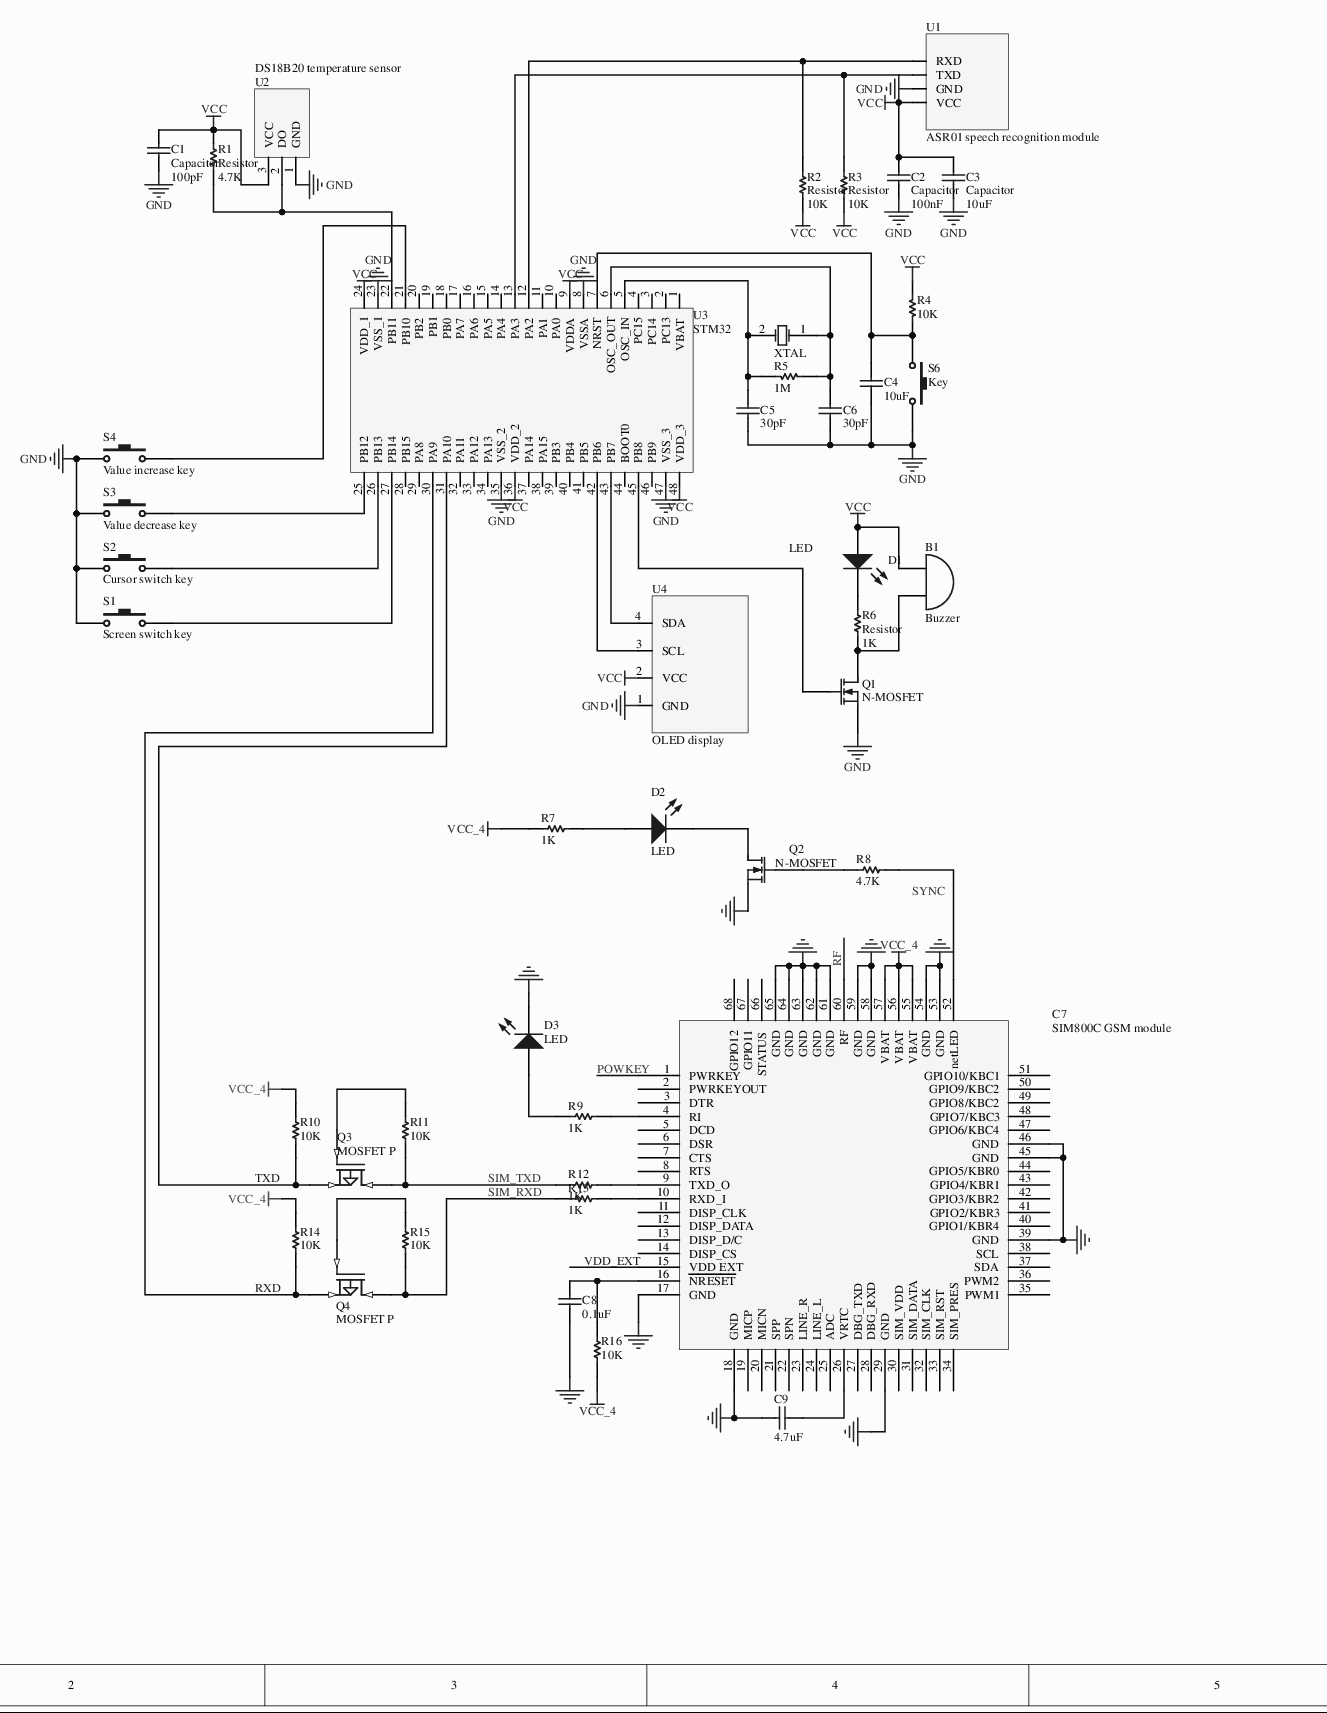
[diagram p0: MISC82701-2.SchDoc, left]
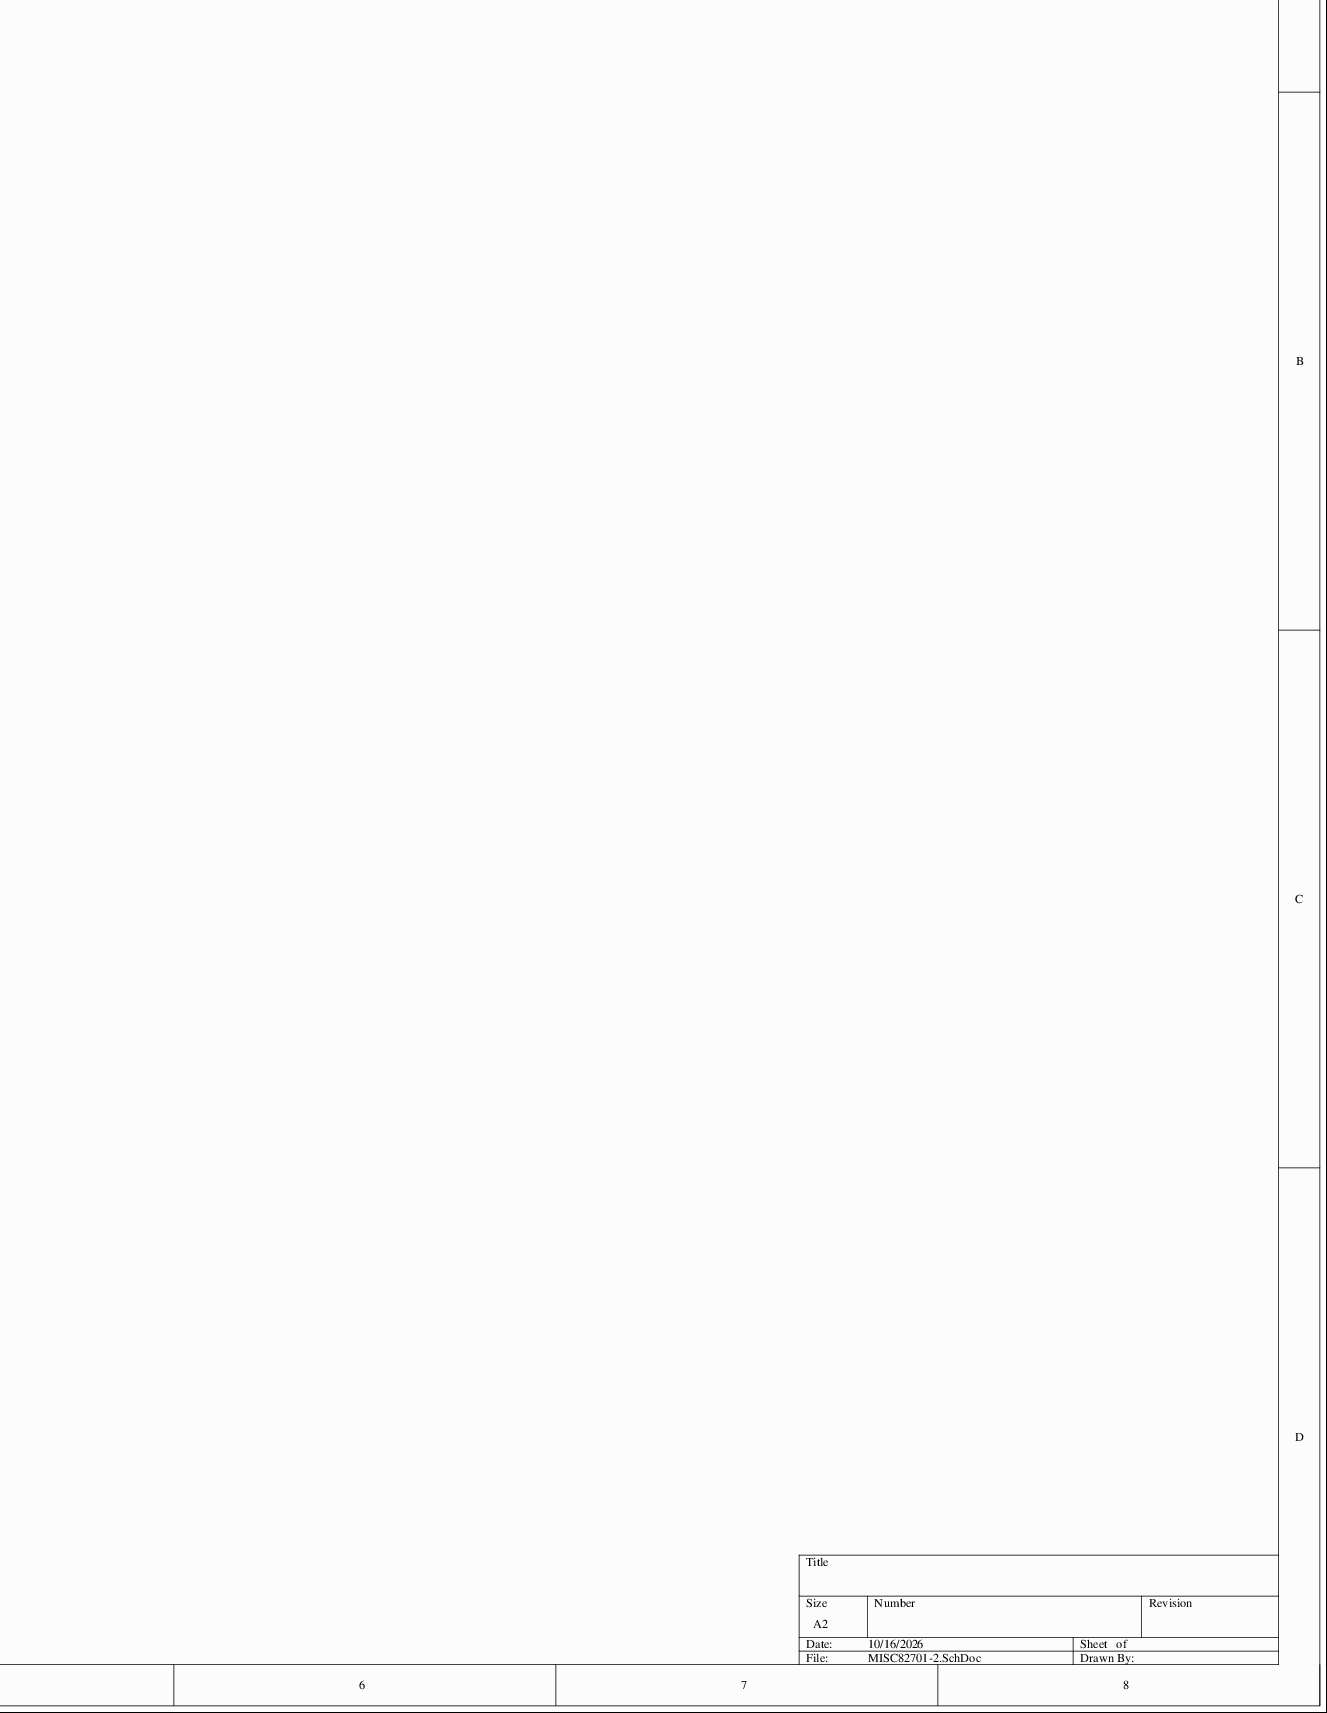
[diagram p1: MISC82701-2.SchDoc, right]
# Altium project MISC82701-7.PrjPcb
1 sheet, 43 parts. Net scope: global (net labels, ports and power ports of the same name join across sheets).
Board file: MISC82701.PcbDoc

## Sheet MISC82701-2.SchDoc
size A2

### Parts
B1  Buzzer  [PIN2]
C1  Capacitor  value 100pF  [0603C]
C2  Capacitor  value 100nF  [0603C]
C3  Capacitor  value 10uF  [0603C]
C4  10uF  [0603C]
C5  value 30pF  [0603C]  (hidden comment: Cap)
C6  value 30pF  [0603C]  (hidden comment: Cap)
C7  SIM800C GSM module  [GSMM_SMD_SIM900A]
C8  value 0.1uF  [0805C]  (hidden comment: Capacitor)
C9  value 4.7uF  [0805C]  (hidden comment: Capacitor)
D1  LED  [3.2X1.6X1.1]
D2  LED  [3.2X1.6X1.1]
D3  LED  [3.2X1.6X1.1]
Q1  N-MOSFET  [SOT23]
Q2  N-MOSFET  [SOT23]
Q3  MOSFET P  [E3]
Q4  MOSFET P  [E3]
R1  Resistor  value 4.7K  [0805R]
R2  Resistor  value 10K  [0805R]
R3  Resistor  value 10K  [0805R]
R4  value 10K  [0805R]  (hidden comment: Res Semi)
R5  value 1M  [0805R]  (hidden comment: Res Semi)
R6  Resistor  value 1K  [0805R]
R7  value 1K  [0805R]  (hidden comment: Resistor)
R8  value 4.7K  [0805R]  (hidden comment: Resistor)
R9  value 1K  [0805R]  (hidden comment: Resistor)
R10  value 10K  [0805R]  (hidden comment: Resistor)
R11  value 10K  [0805R]  (hidden comment: Resistor)
R12  value 1K  [0805R]  (hidden comment: Resistor)
R13  value 1K  [0805R]  (hidden comment: Resistor)
R14  value 10K  [0805R]  (hidden comment: Resistor)
R15  value 10K  [0805R]  (hidden comment: Resistor)
R16  value 10K  [0805R]  (hidden comment: Resistor)
S1  Screen switch key  [四脚轻触开关]
S2  Cursor switch key  [四脚轻触开关]
S3  Value decrease key  [四脚轻触开关]
S4  Value increase key  [四脚轻触开关]
S6  Key  [四脚轻触开关]
U1  ASR01 speech recognition module  [HDR1X4]
U2  DS18B20 temperature sensor  [DS18B20]
U3  STM32  [LQFP48 7X7]
U4  OLED display  [0.96OLED_4P]
Y1  XTAL  [XTAL_US]

### Nets
GND: C1.1 C2.2 C3.2 C4.2 C5.2 C6.2 C7.17(GND) C7.18(GND) C7.29(GND) C7.39(GND) C7.45(GND) C7.46(GND) C7.53(GND) C7.54(GND) C7.58(GND) C7.59(GND) C7.61(GND) C7.62(GND) C7.63(GND) C7.64(GND) C7.65(GND) C8.1 C9.2 D3.2(K) Q1.2(S) Q2.2(S) S1.2 S2.2 S3.2 S4.2 S6.1 U1.2(GND) U2.1(GND) U3.8(VSSA) U3.23(VSS_1) U3.35(VSS_2) U3.47(VSS_3) U4.1(GND)
VCC: B1.1(A) C1.2 C2.1 C3.1 D1.1(A) R1.2 R2.2 R3.2 R4.1 U1.1(VCC) U2.3(VCC) U3.9(VDDA) U3.24(VDD_1) U3.36(VDD_2) U3.48(VDD_3) U4.2(VCC)
VCC_4: C7.55(VBAT) C7.56(VBAT) C7.57(VBAT) R7.2 R10.2 R14.2 R16.1
POWKEY: C7.1(PWRKEY)
RF: C7.60(RF)
RXD: Q4.3(S) R14.1 U3.30(PA9)
SIM_RXD: Q4.2(D) R13.1 R15.1
SIM_TXD: Q3.2(D) R11.1 R12.1
TXD: Q3.3(S) R10.1 U3.31(PA10)
VDD_EXT: C7.15(VDD_EXT)
NetB1_2: B1.2(B) Q1.3(D) R6.2
NetC4_1: C4.1 R4.2 S6.2 U3.7(NRST)
NetC5_1: C5.1 R5.1 U3.5(OSC_IN) Y1.2(OSC2)
NetC6_1: C6.1 R5.2 U3.6(OSC_OUT) Y1.1(OSC1)
NetC7_4: C7.4(RI) R9.2
NetC7_9: C7.9(TXD_O) R12.2
NetC7_10: C7.10(RXD_I) R13.2
NetC7_16: C7.16(~{NRESET}) C8.2 R16.2
NetC7_26: C7.26(VRTC) C9.1
NetC7_52: C7.52(netLED) R8.2
NetD1_2: D1.2(K) R6.1
NetD2_1: D2.1(A) R7.1
NetD2_2: D2.2(K) Q2.3(D)
NetD3_1: D3.1(A) R9.1
NetQ1_1: Q1.1(G) U3.45(PB8)
NetQ2_1: Q2.1(G) R8.1
NetQ3_1: Q3.1(G) R11.2
NetQ4_1: Q4.1(G) R15.2
NetR1_1: R1.1 U2.2(DO) U3.22(PB11)
NetR2_1: R2.1 U1.4(RXD) U3.12(PA2)
NetR3_1: R3.1 U1.3(TXD) U3.13(PA3)
NetS1_1: S1.1 U3.27(PB14)
NetS2_1: S2.1 U3.26(PB13)
NetS3_1: S3.1 U3.25(PB12)
NetS4_1: S4.1 U3.21(PB10)
NetU3_42: U3.42(PB6) U4.3(SCL)
NetU3_43: U3.43(PB7) U4.4(SDA)

Not connected (* = marked no-connect by the designer): C7 2(PWRKEYOUT) 3(DTR) 5(DCD) 6(DSR) 7(CTS) 8(RTS) 11(DISP_CLK) 12(DISP_DATA) 13(DISP_D/C) 14(DISP_CS) 19(MICP) 20(MICN) 21(SPP) 22(SPN) 23(LINE_R) 24(LINE_L) 25(ADC) 27(DBG_TXD) 28(DBG_RXD) 30(SIM_VDD) 31(SIM_DATA) 32(SIM_CLK) 33(SIM_RST) 34(SIM_PRES) 35(PWM1) 36(PWM2) 37(SDA) 38(SCL) 40(GPIO1/KBR4) 41(GPIO2/KBR3) 42(GPIO3/KBR2) 43(GPIO4/KBR1) 44(GPIO5/KBR0) 47(GPIO6/KBC4) 48(GPIO7/KBC3) 49(GPIO8/KBC2) 50(GPIO9/KBC2) 51(GPIO10/KBC1) 66(STATUS) 67(GPIO11) 68(GPIO12); U3 1(VBAT) 2(PC13) 3(PC14) 4(PC15) 10(PA0) 11(PA1) 14(PA4) 15(PA5) 16(PA6) 17(PA7) 18(PB0) 19(PB1) 20(PB2) 28(PB15) 29(PA8) 32(PA11) 33(PA12) 34(PA13) 37(PA14) 38(PA15) 39(PB3) 40(PB4) 41(PB5) 44(BOOT0) 46(PB9)

### Notes on the sheet
- Labels drawn without touching a wire or pin: SYNC

### Library data of the parts
B1 = 蜂鸣器
C1-C3 C8 C9 = 电容: SMD capacitor; Published: 8-Jun-2000; LatestRevisionDate: 17-Jul-2002; LatestRevisionNote: Re-released for DXP Platform.; PackageReference: C1206; Publisher: Altium Limited
C4 = Cap Semi: Capacitor (Semiconductor SIM Model); Published: 8-Jun-2000; LatestRevisionDate: 17-Jul-2002; LatestRevisionNote: Re-released for DXP Platform.; PackageReference: C1206; Value: 10uF; Publisher: Altium Limited
C5 C6 = Cap: Capacitor; Published: 8-Jun-2000; LatestRevisionDate: 17-Jul-2002; LatestRevisionNote: Re-released for DXP Platform.; PackageReference: RAD-0.3; Publisher: Altium Limited
C7 = SIM 900A
D1-D3 = LED灯
Q1 Q2 = SI2302: MOSFET
R1-R3 R6-R16 = 电阻: SMD resistor; Published: 8-Jun-2000; LatestRevisionDate: 17-Jul-2002; LatestRevisionNote: Re-released for DXP Platform.; PackageReference: AXIAL-0.5; Publisher: Altium Limited
R4 R5 = Res Semi: Semiconductor Resistor; Published: 8-Jun-2000; LatestRevisionDate: 17-Jul-2002; LatestRevisionNote: Re-released for DXP Platform.; PackageReference: AXIAL-0.5; Publisher: Altium Limited
S1-S4 S6 = 按键
U1 = HC-05蓝牙模块_1: HC-05 Bluetooth module
U2 = DS18B20: Temperature sensor
U3 = STM32F103C8T6_2
U4 = OLED显示器2
Y1 = XTAL: Crystal Oscillator; Published: 8-Jun-2000; LatestRevisionDate: 17-Jul-2002; LatestRevisionNote: Re-released for DXP Platform.; PackageReference: R38; Publisher: Altium Limited